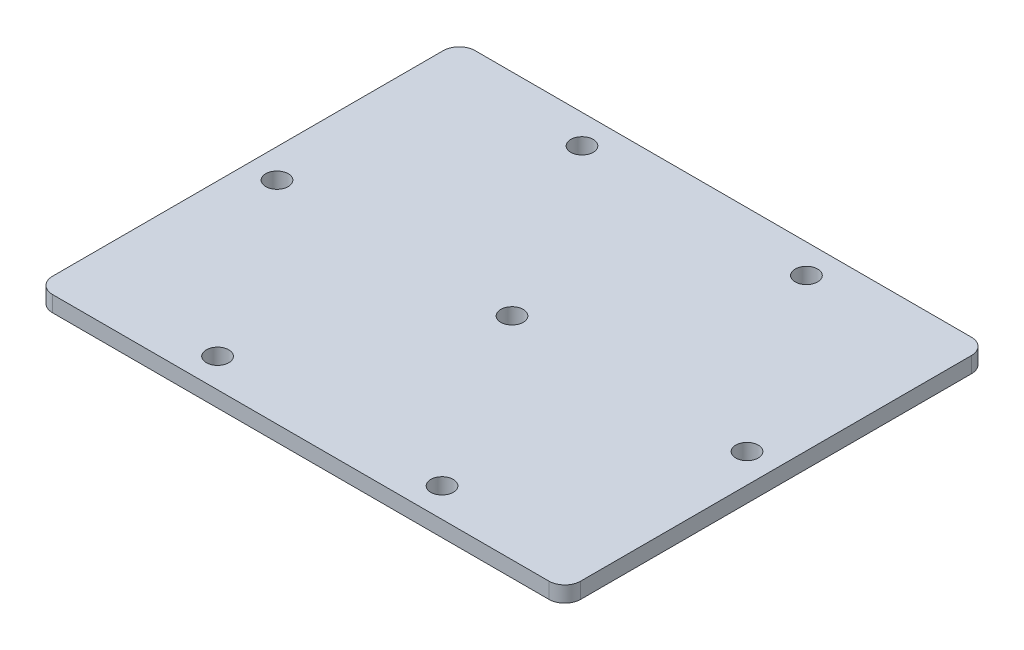
from build123d import *

# Parameters (mm, degrees)
SKETCH1_W           = 200
SKETCH1_H           = 160
BOSS_EXTRUDE1_DEPTH = 6
FILLET1_R           = 6
M10_TAPPED_HOLE1_D  = 8.5


with BuildPart() as part:
    # Sketch1 → Boss-Extrude1 (new body)
    with BuildSketch(Plane(origin=(0, 0, 0), x_dir=(1, 0, 0), z_dir=(0, 1, 0))):
        Rectangle(SKETCH1_W, SKETCH1_H)
    extrude(amount=BOSS_EXTRUDE1_DEPTH)

    # Fillet1
    fillet1_edges = [part.edges().sort_by_distance(p)[0] for p in [
        (100, 3, 80),
        (-100, 3, 80),
        (-100, 3, -80),
        (100, 3, -80),
    ]]
    fillet(fillet1_edges, radius=FILLET1_R)

    # M10 Tapped Hole1 (through all)
    with Locations(Plane(origin=(0, 6, 0), x_dir=(1, 0, 0), z_dir=(0, 1, 0))):
        with Locations((0, 0), (42.5, 69), (-42.5, 69), (-89, 0), (89, 0), (42.5, -69), (-42.5, -69)):
            Hole(M10_TAPPED_HOLE1_D / 2)


solid = part.part
